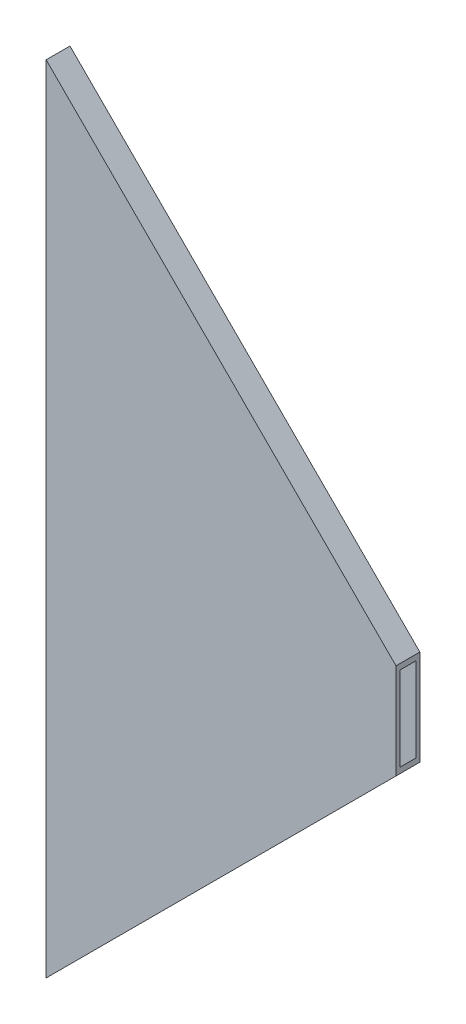
from build123d import *

# Parameters (mm, degrees)
BOSS_EXTRUDE1_DEPTH   = 30
SKETCH2_W             = 120
SKETCH2_H             = 120
CUT_EXTRUDE1_DEPTH    = 30
SKETCH3_W             = 90
SKETCH3_H             = 50
CUT_EXTRUDE2_DEPTH    = 7
SHELL1_T              = -5
M4_TAPPED_HOLE1_D     = 3.3
M4_TAPPED_HOLE1_DEPTH = 10.1
M4_TAPPED_HOLE1_TIP   = 0.991420021


with BuildPart() as part:
    # Sketch1 → Boss-Extrude1 (new body)
    with BuildSketch(Plane.XY):
        Polygon((-500, 500), (0, 0), (-500, -500), align=None)
    extrude(amount=BOSS_EXTRUDE1_DEPTH)

    # Sketch2 → Cut-Extrude1 (cut)
    with BuildSketch(Plane.XY.offset(30)):
        Rectangle(SKETCH2_W, SKETCH2_H)
    extrude(amount=-CUT_EXTRUDE1_DEPTH, mode=Mode.SUBTRACT)

    # Sketch3 → Cut-Extrude2 (cut)
    with BuildSketch(Plane.ZY.offset(500)):
        with Locations((-20, 325)):
            Rectangle(SKETCH3_W, SKETCH3_H)
        with Locations((-20, -325)):
            Rectangle(SKETCH3_W, SKETCH3_H)
    extrude(amount=-CUT_EXTRUDE2_DEPTH, mode=Mode.SUBTRACT)

    # Shell1
    shell1_openings = [part.faces().sort_by_distance(p)[0] for p in [
        (-60, 0, 15),
    ]]
    offset(amount=SHELL1_T, openings=shell1_openings, kind=Kind.INTERSECTION)

    # M4 Tapped Hole1
    with Locations(Plane.ZY.offset(493)):
        with Locations((17.5, 335), (17.5, 315), (17.5, -315), (17.5, -335)):
            Hole(M4_TAPPED_HOLE1_D / 2, depth=M4_TAPPED_HOLE1_DEPTH)
            with Locations((0, 0, -(M4_TAPPED_HOLE1_DEPTH + M4_TAPPED_HOLE1_TIP / 2))):  # 118° drill point
                Cone(0, M4_TAPPED_HOLE1_D / 2, M4_TAPPED_HOLE1_TIP, mode=Mode.SUBTRACT)


solid = part.part
